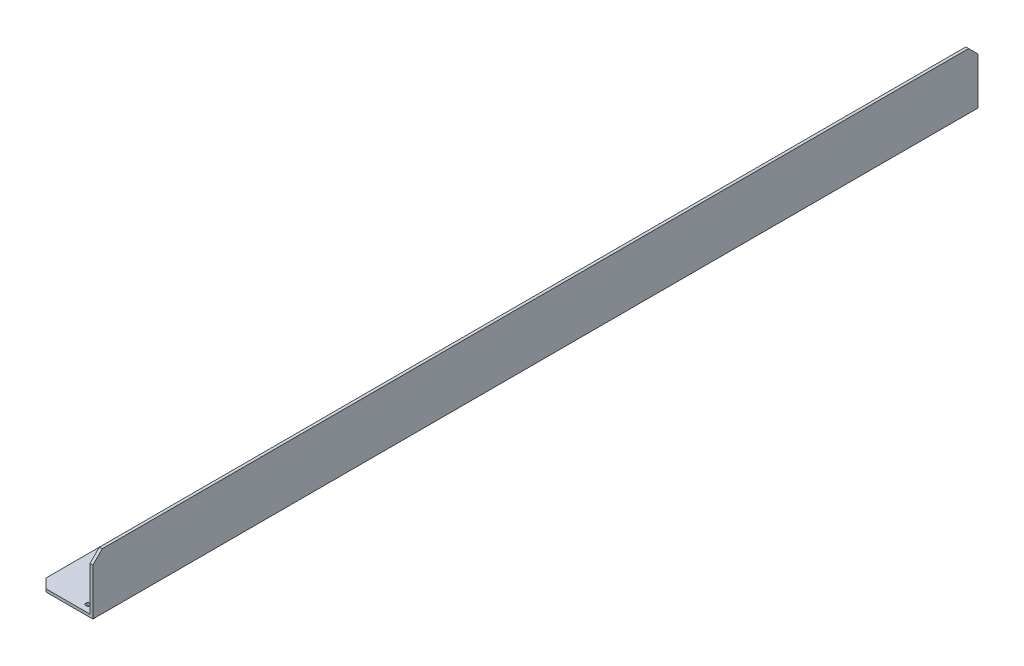
SolidWorks part; units mm, degrees
material "6061Al"
ref_plane "前视基准面" through (0, 0, 0) normal (0, 0, 1) x (1, 0, 0)
ref_plane "上视基准面" through (0, 0, 0) normal (0, 1, 0) x (1, 0, 0)
ref_plane "右视基准面" through (0, 0, 0) normal (1, 0, 0) x (0, 0, -1)
sketch "草图1" plane through (0, 0, 0) normal (0, 0, 1) x (1, 0, 0)
  line L0 (0, 0) -> (60, 0)
  line L1 (60, 0) -> (60, 60)
  line L2 (60, 60) -> (57, 60)
  line L3 (57, 60) -> (57, 3)
  line L4 (57, 3) -> (0, 3)
  line L5 (0, 3) -> (0, 0)
  dimension "D1" = 3
  dimension "D2" = 3
  dimension "D3" = 60
  dimension "D4" = 60
extrude "凸台-拉伸1" add sketch "草图1" along normal mid plane 945
hole_wizard "M4 间隙孔1" positions "草图4" profile "草图5" hole size "M4" standard "ISO" end condition through all
sketch "草图4" plane through (0, 3, 0) normal (0, 1, 0) x (1, 0, 0)
  line L0 (0, 0) -> (47, 0) construction
  line L2 (57, -472.5) -> (57, 472.5) construction
  line L3 (47, 0) -> (47, 232.25) construction
  line L4 (57, 472.5) -> (0, 472.5) construction
  point P0 (47, 0)
  point P12 (47, 232.25)
  point P13 (47, 464.5)
  point P16 (47, -464.5)
  point P17 (47, -232.25)
  point P21 (47, 449.5)
  point P24 (47, -449.5)
  dimension "D1" = 10
  dimension "D3" = 8
  dimension "D4" = 15
  dimension "D2" = 3
sketch "草图5" plane through (47, 3, 0) normal (1, 0, 0) x (0, 0, 1)
  line L0 (0, 0) -> (0, 3)
  line L1 (0, 3) -> (2.4, 3)
  line L2 (2.4, 3) -> (2.4, 0)
  line L5 (2.4, 0) -> (0, 0)
  line L11 (0, -6.35) -> (0, 107.95) construction
  dimension "通孔孔直径" = 4.8
  dimension "通孔孔深度" = 3
chamfer "倒角1" distance 10 angle 45 4 edges at (58.5, 60, -472.5) (0, 1.5, -472.5) (58.5, 60, 472.5) (0, 1.5, 472.5)
hole_wizard "M5 螺纹孔1" positions "草图6" profile "草图7" tap size "M5" standard "ISO" end condition up to next
sketch "草图6" plane through (0, 3, 0) normal (0, 1, 0) x (1, 0, 0)
  line L0 (57, 472.5) -> (10, 472.5) construction
  line L1 (0, -462.5) -> (0, 462.5) construction
  line L2 (9.75, 373.7) -> (39.75, 373.7) construction
  point P0 (9.75, 373.7)
  point P3 (39.75, 373.7)
  point P6 (24.75, 358.7)
  point P24 (9.75, 358.7)
  point P26 (39.75, 358.7)
  point P28 (24.75, 373.7)
  dimension "D1" = 15
  dimension "D2" = 15
  dimension "D3" = 15
  dimension "D4" = 113.8
  dimension "D5" = 24.75
sketch "草图7" plane through (9.75, 3, -373.7) normal (1, 0, 0) x (0, 0, 1)
  line L0 (0, 0) -> (0, 3)
  line L1 (0, 3) -> (2.1, 3)
  line L2 (2.1, 3) -> (2.1, 0)
  line L5 (2.1, 0) -> (0, 0)
  line L11 (0, -6.35) -> (0, 107.95) construction
  dimension "通孔螺纹孔钻头直径" = 4.2
  dimension "通孔螺纹孔钻头深度" = 3
cosmetic thread "孔螺蚊线1" parameters "D2"=5
cosmetic thread "孔螺蚊线2" parameters "D2"=5
cosmetic thread "孔螺蚊线3" parameters "D2"=5
cosmetic thread "孔螺蚊线4" parameters "D2"=5
cosmetic thread "孔螺蚊线5" parameters "D2"=5
cosmetic thread "孔螺蚊线6" parameters "D2"=5
